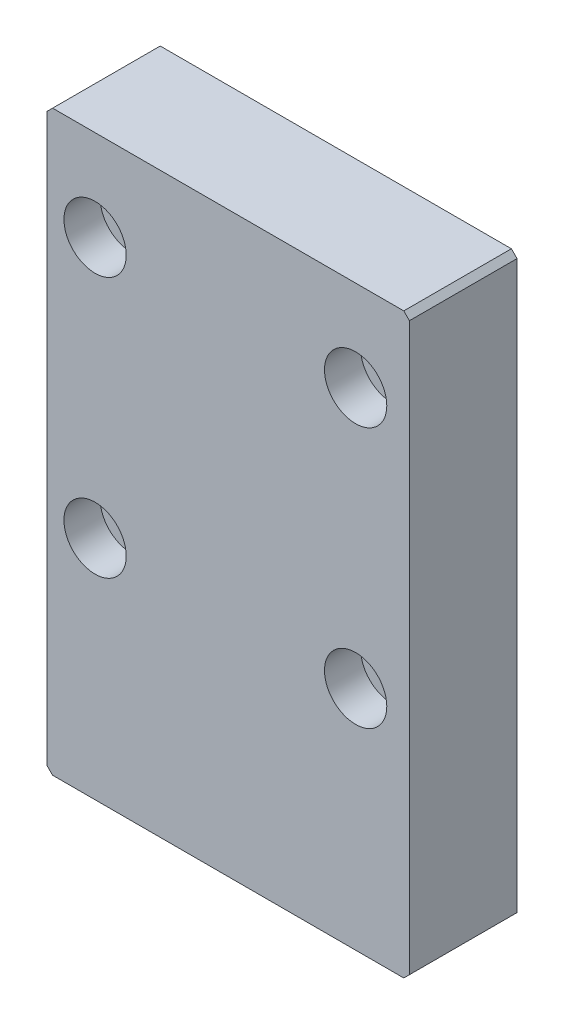
SolidWorks part; units mm, degrees
material "Al6061"
ref_plane "Front" through (0, 0, 0) normal (0, 0, 1) x (1, 0, 0)
ref_plane "Top" through (0, 0, 0) normal (0, 1, 0) x (1, 0, 0)
ref_plane "Right" through (0, 0, 0) normal (1, 0, 0) x (0, 0, -1)
sketch "草图15" plane through (0, 0, 0) normal (0, 0, 1) x (1, 0, 0)
  line L1 (-18.9278, 29.277) -> (25.0722, 29.277)
  line L2 (-18.9278, 29.277) -> (-18.9278, -90.723)
  line L3 (-18.9278, -90.723) -> (25.0722, -90.723)
  line L4 (25.0722, 29.277) -> (25.0722, -90.723)
  dimension "D1" = 44
  dimension "D2" = 120
extrude "凸台-拉伸1" add sketch "草图15" along normal blind 19
hole_wizard "打孔尺寸根据内六角圆柱头螺钉的类型1" positions "草图17" profile "草图16" counterbore size "M4" standard "Gb"
sketch "草图17" plane through (0, 0, 10) normal (0, 0, 1) x (1, 0, 0)
  line L0 (-18.9278, 29.277) -> (-18.9278, -90.723) construction
  line L1 (25.0722, 29.277) -> (-18.9278, 29.277) construction
  point P0 (-13.9278, -6.723)
  point P2 (20.0722, -6.723)
  point P4 (20.0722, -48.723)
  point P6 (-13.9278, -48.723)
  dimension "D1" = 34
  dimension "D2" = 42
  dimension "D3" = 5
  dimension "D4" = 36
sketch "草图16" plane through (-13.9278, -6.723, 10) normal (1, 0, 0) x (0, -1, 0)
  line L0 (0, 0) -> (0, 10)
  line L1 (0, 10) -> (2.25, 10)
  line L3 (2.25, 10) -> (2.25, 4.6)
  line L4 (2.25, 4.6) -> (4, 4.6)
  line L5 (4, 4.6) -> (4, 0)
  line L7 (4, 0) -> (0, 0)
  line L11 (0, -6.35) -> (0, 107.95) construction
  dimension "通孔孔直径" = 4.5
  dimension "通孔孔深度" = 10
  dimension "柱形沉头孔直径" = 8
  dimension "柱形沉头孔深度" = 4.6
hole_wizard "M4 螺纹孔2" positions "草图19" profile "草图18" tap size "M4" standard "Iso"
sketch "草图19" plane through (0, 0, 0) normal (0, 0, -1) x (-1, 0, 0)
  line L1 (18.9278, 29.277) -> (18.9278, -90.723) construction
  line L2 (-25.0722, -90.723) -> (-25.0722, 29.277) construction
  line L3 (18.9278, -90.723) -> (-25.0722, -90.723) construction
  point P0 (-3.0722, 2.277)
  point P3 (-3.0722, -26.723)
  point P6 (-3.0722, -65.723)
  dimension "D1" = 22
  dimension "D2" = 22
  dimension "D3" = 39
  dimension "D4" = 29
  dimension "D5" = 25
cosmetic thread "孔螺蚊线3" parameters "D1"=8, "D2"=4
cosmetic thread "孔螺蚊线4" parameters "D1"=8, "D2"=4
cosmetic thread "孔螺蚊线5" parameters "D1"=8, "D2"=4
sketch "草图18" plane through (3.0722, 2.277, 0) normal (1, 0, 0) x (0, 1, 0)
  line L0 (0, 0) -> (0, 12.4914)
  line L1 (0, 12.4914) -> (1.65, 11.5)
  line L2 (1.65, 11.5) -> (1.65, 0)
  line L5 (1.65, 0) -> (0, 0)
  line L10 (0, 12.4914) -> (-1.65, 11.5) construction
  line L11 (0, -6.35) -> (0, 107.95) construction
  dimension "螺纹孔钻头直径" = 3.3
  dimension "螺纹孔钻头深度" = 11.5
  dimension "导头角度" = 118
sketch "草图21" plane through (0, 0, 19) normal (0, 0, 1) x (1, 0, 0)
  line L0 (-18.9278, 11.277) -> (25.0722, 11.277)
  line L1 (25.0722, 11.277) -> (25.0722, 29.277)
  line L2 (25.0722, 29.277) -> (-18.9278, 29.277)
  line L3 (-18.9278, 29.277) -> (-18.9278, 11.277)
extrude "切除-拉伸4" cut sketch "草图21" against normal blind 19
hole_wizard "M4 螺纹孔1" positions "草图23" profile "草图22" tap size "M4" standard "Iso"
sketch "草图23" plane through (0, 0, 0) normal (0, 0, -1) x (-1, 0, 0)
  line L0 (-25.0722, -90.723) -> (-25.0722, 11.277) construction
  line L1 (18.9278, 11.277) -> (-25.0722, 11.277) construction
  point P0 (-13.0722, 7.277)
  point P2 (6.9278, 7.277)
  dimension "D1" = 20
  dimension "D2" = 12
  dimension "D3" = 4
sketch "草图22" plane through (13.0722, 7.277, 0) normal (1, 0, 0) x (0, 1, 0)
  line L0 (0, 0) -> (0, 11.0914)
  line L1 (0, 11.0914) -> (1.65, 10.1)
  line L2 (1.65, 10.1) -> (1.65, 0)
  line L5 (1.65, 0) -> (0, 0)
  line L10 (0, 11.0914) -> (-1.65, 10.1) construction
  line L11 (0, -6.35) -> (0, 107.95) construction
  dimension "螺纹孔钻头直径" = 3.3
  dimension "螺纹孔钻头深度" = 10.1
  dimension "导头角度" = 118
cosmetic thread "孔螺蚊线1" parameters "D1"=8, "D2"=4
cosmetic thread "孔螺蚊线2" parameters "D1"=8, "D2"=4
chamfer "倒角1" distance 1 angle 45 4 edges at (25.0722, -90.723, 9.5) (-18.9278, -90.723, 9.5) (25.0722, 11.277, 9.5) (-18.9278, 11.277, 9.5)
sketch "草图24" plane through (0, 0, 19) normal (0, 0, 1) x (1, 0, 0)
  line L0 (-17.9278, -90.723) -> (24.0722, -90.723) construction
  line L1 (-28.9278, 11.277) -> (-15.1565, 11.277)
  line L2 (-28.9278, 11.277) -> (-28.9278, -90.723)
  line L3 (-28.9278, -90.723) -> (-15.1565, -90.723)
  line L4 (35.0722, 11.277) -> (35.0722, -90.723)
  line L5 (-18.9278, 10.277) -> (-18.9278, -89.723) construction
  line L7 (-17.9278, 11.277) -> (24.0722, 11.277) construction
  line L8 (22.0397, 11.277) -> (22.0397, -90.723)
  line L9 (-15.1565, 11.277) -> (-15.1565, -90.723)
  line L10 (22.0397, 11.277) -> (35.0722, 11.277)
  line L11 (22.0397, -90.723) -> (35.0722, -90.723)
  dimension "D1" = 64
  dimension "D2" = 10
extrude "凸台-拉伸2" add sketch "草图24" against normal up to vertex (19 mm away)
hole_wizard "M6 六角凹头螺钉的柱形沉头孔1" positions "草图26" profile "草图25" counterbore size "M6" standard "Iso" end condition through all
sketch "草图26" plane through (0, 0, 19) normal (0, 0, 1) x (1, 0, 0)
  line L0 (-28.9278, 11.277) -> (35.0722, 11.277) construction
  point P0 (-20.4278, -4.723)
  point P2 (25.5722, -4.723)
  point P4 (25.5722, -50.703)
  point P6 (-20.4278, -50.723)
  dimension "D1" = 16
  dimension "D2" = 46
  dimension "D3" = 46
sketch "草图25" plane through (-20.4278, -4.723, 19) normal (1, 0, 0) x (0, -1, 0)
  line L0 (0, 0) -> (0, 19)
  line L1 (0, 19) -> (3.3, 19)
  line L3 (3.3, 19) -> (3.3, 6.4)
  line L4 (3.3, 6.4) -> (5.5, 6.4)
  line L5 (5.5, 6.4) -> (5.5, 0)
  line L7 (5.5, 0) -> (0, 0)
  line L11 (0, -6.35) -> (0, 107.95) construction
  dimension "通孔孔直径" = 6.6
  dimension "通孔孔深度" = 19
  dimension "柱形沉头孔直径" = 11
  dimension "柱形沉头孔深度" = 6.4
chamfer "倒角2" distance 1 angle 45 4 edges at (35.0722, -90.723, 9.5) (-28.9278, -90.723, 9.5) (35.0722, 11.277, 9.5) (-28.9278, 11.277, 9.5)
